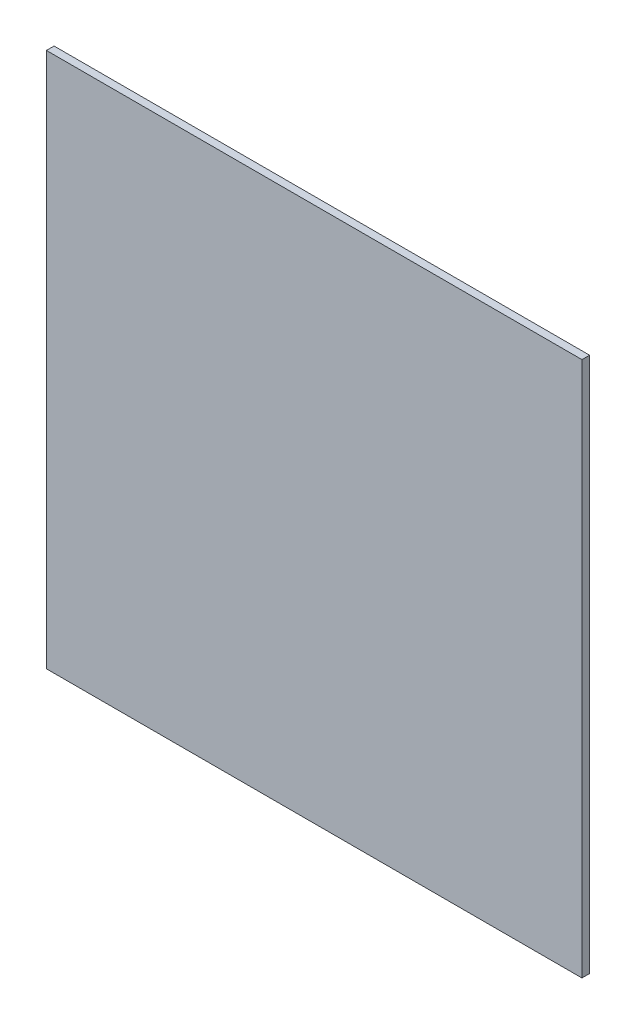
SolidWorks part; units mm, degrees
ref_plane "前视基准面" through (0, 0, 0) normal (0, 0, 1) x (1, 0, 0)
ref_plane "上视基准面" through (0, 0, 0) normal (0, 1, 0) x (1, 0, 0)
ref_plane "右视基准面" through (0, 0, 0) normal (1, 0, 0) x (0, 0, -1)
other "Configuration Table"
sketch "草图1" plane through (0, 0, 0) normal (0, 0, 1) x (1, 0, 0)
  line L0 (-140, -140) -> (140, -140)
  line L1 (140, -140) -> (140, 140)
  line L2 (140, 140) -> (-140, 140)
  line L3 (-140, 140) -> (-140, -140)
  point P0 (0, 0)
  dimension "D1" = 140
  dimension "D2" = 280
  dimension "D3" = 140
  dimension "D4" = 280
extrude "凸台-拉伸1" add sketch "草图1" against normal mid plane 4
